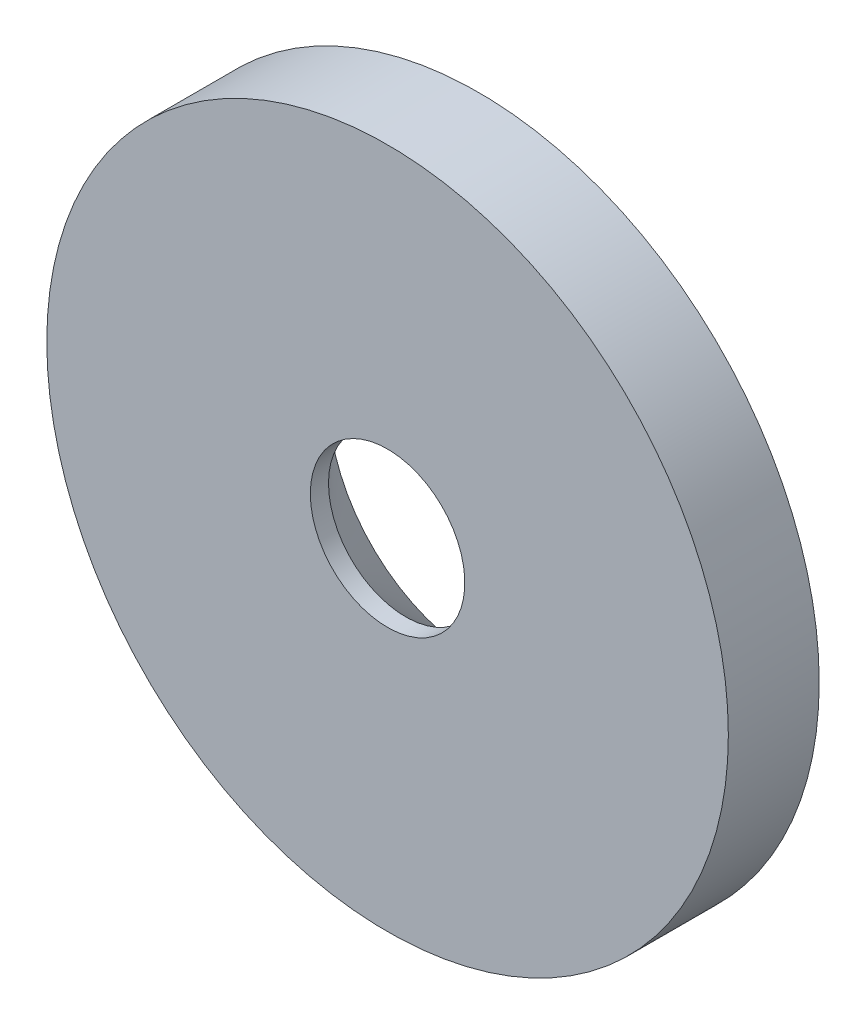
SolidWorks part; units mm, degrees
ref_plane "前视基准面" through (0, 0, 0) normal (0, 0, 1) x (1, 0, 0)
ref_plane "上视基准面" through (0, 0, 0) normal (0, 1, 0) x (1, 0, 0)
ref_plane "右视基准面" through (0, 0, 0) normal (1, 0, 0) x (0, 0, -1)
sketch "草图1" plane through (0, 0, 0) normal (0, 0, 1) x (1, 0, 0)
  circle A0 centre (0, 0) radius 7.5
  circle A1 centre (0, 0) radius 1
  dimension "D1" = 15
  dimension "D2" = 2
extrude "凸台-拉伸1" add sketch "草图1" along normal blind 2
sketch "草图4" plane through (0, 0, 0) normal (0, 0, -1) x (-1, 0, 0)
  point P0 (0, 0)
hole_wizard "M3 开槽沉头木螺钉的锥形沉头孔1" positions "草图4" profile "草图5" countersink size "M3" standard "GB" end condition through all
sketch "草图5" plane through (0, 0, 0) normal (1, 0, 0) x (0, 1, 0)
  line L0 (0, 0) -> (0, 2)
  line L1 (0, 2) -> (1.7, 2)
  line L2 (1.7, 2) -> (1.7, 1.6)
  line L3 (1.7, 1.6) -> (3.3, 0)
  line L5 (3.3, 0) -> (0, 0)
  line L6 (-1.7, 1.6) -> (-3.3, 0) construction
  line L11 (0, -6.35) -> (0, 107.95) construction
  dimension "通孔孔直径" = 3.4
  dimension "通孔孔深度" = 2
  dimension "近端锥形沉头孔直径" = 6.6
  dimension "近端锥形沉头孔角度" = 90
